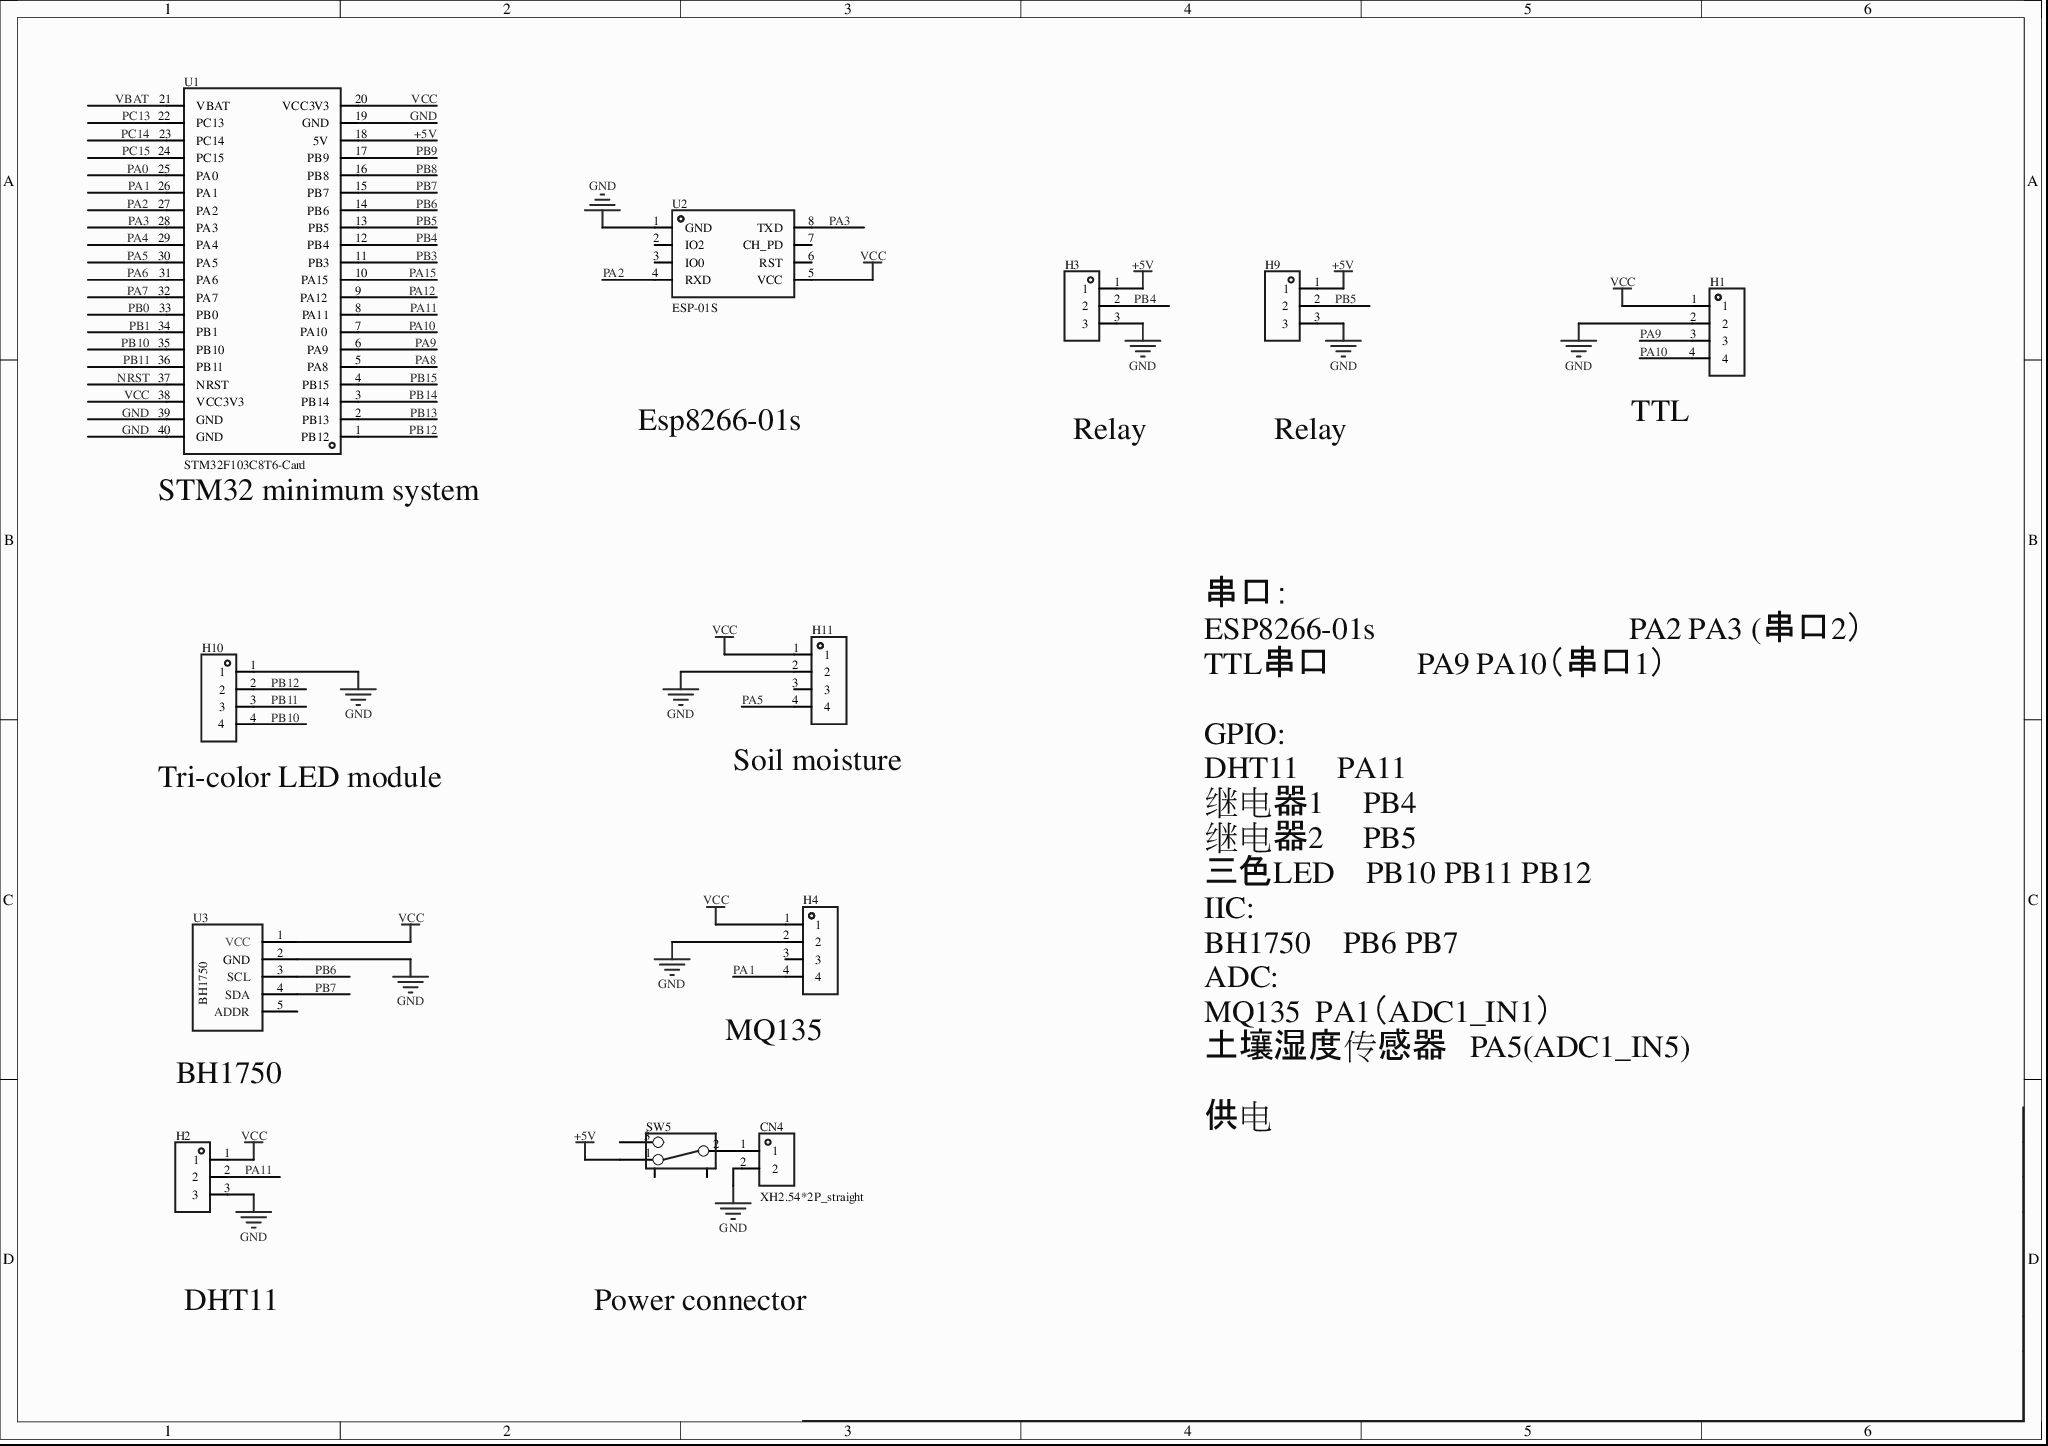
[diagram p0: MISC79011-3.schdoc]
# Altium project MISC79011-2.PrjPcb
1 sheet, 12 parts. Net scope: global (net labels, ports and power ports of the same name join across sheets).
Board file: MISC79011.pcbdoc

## Sheet MISC79011-3.schdoc
size 297 x 209 mm; Version: V1.0; @Project Name: MISC79011; @Page Count: 1; @Update Date: 2026-05-03; @Create Date: 2026-05-03; @Schematic Name: MISC79011; @Page No: 1; @Create Time: 23:22:16; @Update Time: 17:32:40; @Board Name: MISC79011

### Parts
CN4  XH2.54*2P_straight  [CONN-TH_2P-P2.50-XH2.54-2P]
H1  (no value)  [HDR-TH_4P-P2.54-V-F]
H2  (no value)  [HDR-TH_3P-P2.54-V-F]
H3  (no value)  [HDR-TH_3P-P2.54-V-F]
H4  (no value)  [HDR-TH_4P-P2.54-V-F]
H9  (no value)  [HDR-TH_3P-P2.54-V-F]
H10  (no value)  [HDR-TH_4P-P2.54-V-F]
H11  (no value)  [HDR-TH_4P-P2.54-V-F]
SW5  (no value)  [拨动开关]
U1  STM32F103C8T6-Card  [CONN-TH_L53.3-W22.9_STM32F103C8T6-CARD]
U2  ESP-01S  [WIFIM-TH_ESP-01S]
U3  (no value)  [BH1750光照传感器]

### Nets
+5V: H3.1 H9.1 SW5.1 U1.18(5V)
GND: CN4.2 H1.2 H2.3 H3.3 H4.2 H9.3 H10.1 H11.2 U1.19(GND) U1.39(GND) U1.40(GND) U2.1(GND) U3.2(GND)
VCC: H1.1 H2.1 H4.1 H11.1 U1.20(VCC3V3) U1.38(VCC3V3) U2.5(VCC) U3.1(VCC)
NRST: U1.37(NRST)
PA0: U1.25(PA0)
PA1: H4.4 U1.26(PA1)
PA2: U1.27(PA2) U2.4(RXD)
PA3: U1.28(PA3) U2.8(TXD)
PA4: U1.29(PA4)
PA5: H11.4 U1.30(PA5)
PA6: U1.31(PA6)
PA7: U1.32(PA7)
PA8: U1.5(PA8)
PA9: H1.3 U1.6(PA9)
PA10: H1.4 U1.7(PA10)
PA11: H2.2 U1.8(PA11)
PA12: U1.9(PA12)
PA15: U1.10(PA15)
PB0: U1.33(PB0)
PB1: U1.34(PB1)
PB3: U1.11(PB3)
PB4: H3.2 U1.12(PB4)
PB5: H9.2 U1.13(PB5)
PB6: U1.14(PB6) U3.3(SCL)
PB7: U1.15(PB7) U3.4(SDA)
PB8: U1.16(PB8)
PB9: U1.17(PB9)
PB10: H10.4 U1.35(PB10)
PB11: H10.3 U1.36(PB11)
PB12: H10.2 U1.1(PB12)
PB13: U1.2(PB13)
PB14: U1.3(PB14)
PB15: U1.4(PB15)
PC13: U1.22(PC13)
PC14: U1.23(PC14)
PC15: U1.24(PC15)
VBAT: U1.21(VBAT)
NetCN4_1: CN4.1 SW5.2

Not connected (* = marked no-connect by the designer): H4 3; H11 3; SW5 3 4 5; U2 2(IO2)* 3(IO0)* 6(RST)* 7(CH_PD)*; U3 5(ADDR)

### Notes on the sheet
- Esp8266-01s
- (near H1) TTL
- (near U1) STM32 minimum system
- Relay
- 串口：
  ESP8266-01s  		PA2 PA3 (串口2）
  TTL串口           PA9 PA10（串口1）
  GPIO:
  DHT11     PA11
  继电器1     PB4
  继电器2     PB5
  三色LED    PB10 PB11 PB12
  IIC:
  BH1750    PB6 PB7
  ADC:
  MQ135  PA1（ADC1_IN1）
  土壤湿度传感器   PA5(ADC1_IN5)
  供电
- (near H11) Soil moisture
- (near H10) Tri-color LED module
- (near H4) MQ135
- BH1750
- DHT11
- Power connector

### Library data of the parts
CN4 = XH2.54*2P_直插: 3D Model: 325c595e30db4df8abe76612dd40b0fa0819f05c4eef4c71ace90d822a990e87; 3D Model Transform: 295.275,228.346,0,180,0,0,-0.002,-20.079,-137.795; AddInBom: yes; Device: XH2.54*2P_straight; Symbol: XH2.54*2P_straight; LCSC Part Name: XH2.54*2P_直插; Supplier Part: C9900008615; Manufacturer Part: XH2.54*2P_直插; Supplier Footprint: XH2.54_2P; JLCPCB Part Class: Extended Part; Supplier: LCSC; FootprintName: CONN-TH_2P-P2.50-XH2.54-2P; ConvertToPcb: yes; ModelName: CONN-TH_2P-P2.50-XH2.54-2P
H1 H11 = HDR-F_2.54_1x4P: Symbol: 2.54-1*4P female; 3D Model: d187812051054f85879fcaa51a310d8e0819f05c4eef4c71ace90d822a990e87; 3D Model Transform: 419.6842,98.464,0,0,0,0,0,0,-118.11; ConvertToPcb: yes; Device: HDR-F_2.54_1x4P; Supplier Part: C2718488; Supplier Footprint: 插件; FootprintName: HDR-TH_4P-P2.54-V-F; AddInBom: yes; ModelName: HDR-TH_4P-P2.54-V-F
H2 H3 H9 = HDR-F_2.54_1x3P: Symbol: PM254V-11-03-H85; 3D Model: f3b3cc5aae9641bf9e56fc160cef875b; 3D Model Transform: 299.9994,100,0,0,0,0,0,0,-118.11; ConvertToPcb: yes; ModelName: HDR2.54-F-LI-1X3P; Device: HDR-F_2.54_1x3P; Supplier Part: C541850; Supplier Footprint: 插件; FootprintName: HDR-TH_3P-P2.54-V-F; AddInBom: yes
H4 H10 = HDR-F_2.54_1x4P: Symbol: 2.54-1*4P female; ConvertToPcb: yes; ModelId: d187812051054f85879fcaa51a310d8e0819f05c4eef4c71ace90d822a990e87; ModelTransform: 419.6842,98.464,0,0,0,0,0,0,-118.11; Device: HDR-F_2.54_1x4P; FootprintName: HDR-TH_4P-P2.54-V-F; AddInBom: yes; SupplierPart: C2718488; Supplier Footprint: 插件; ModelName: HDR-TH_4P-P2.54-V-F
SW5 = 拨动开关_正: Device: Toggle switch_upright; Symbol: Toggle switch; ConvertToPcb: yes; ModelId: 4321fe59a4074cbfb4989553f297c68f0819f05c4eef4c71ace90d822a990e87; ModelName: SW-TH_SS-12D02-VG4; ModelTransform: 370.09,208.7,472.35,0,0,0,0,0,-110; FootprintName: Toggle switch; AddInBom: yes; Supplier Footprint: 插件
U1 = STM32F103C8T6-Card: AddInBom: yes; Device: STM32F103C8T6-Card; Symbol: STM32F103C8T6-CARD; FootprintName: CONN-TH_L53.3-W22.9_STM32F103C8T6-CARD; LCSC Part Name: STM32F103C8T6-Card; SupplierPart: C9900077949; ManufacturerPart: STM32F103C8T6-Card; Supplier Footprint: 插件; Supplier: LCSC; ConvertToPcb: yes
U2 = ESP-01S_C111009: 3D Model: eb7175da78ae48b3b1568cfe3027405f0819f05c4eef4c71ace90d822a990e87; 3D Model Transform: 582.676,976.37608,0,0,0,0,0,388.346,-118.11; AddInBom: yes; Symbol: ESP-01S; Device: ESP-01S_C111009; LCSC Part Name: ESP-01S; Supplier Part: C111009; Manufacturer Part: ESP-01S; Supplier Footprint: -; JLCPCB Part Class: Extended Part; Supplier: LCSC; ConvertToPcb: yes; FootprintName: WIFIM-TH_ESP-01S; ModelName: WIFIM-TH_ESP-01S
U3 = BH1750光照传感器: Symbol: BH1750 light sensor; AddInBom: yes; Device: BH1750 light sensor; ConvertToPcb: yes; FootprintName: BH1750 light sensor